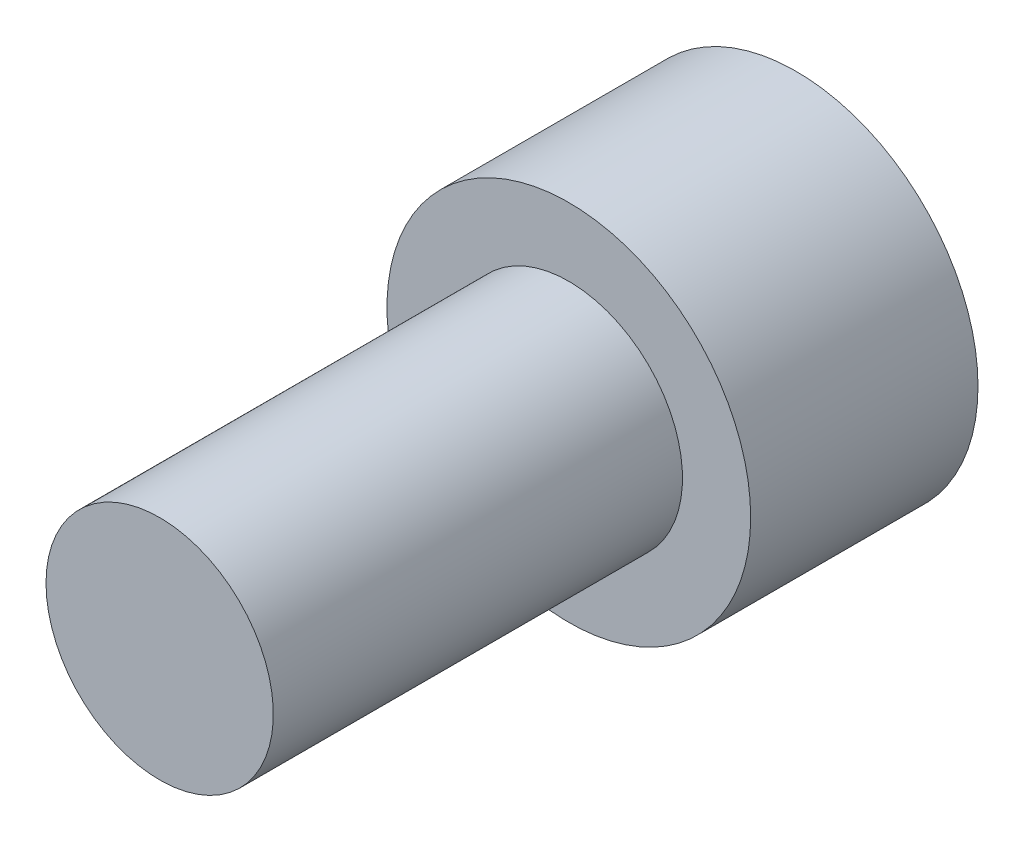
from build123d import *

# Parameters (mm, degrees)
SKETCH_1_R      = 20
EXTRUDE_1_DEPTH = 25
SKETCH_2_R      = 12.5
EXTRUDE_2_DEPTH = 45


with BuildPart() as part:
    # 草图1 → 凸台-拉伸1 (new body)
    with BuildSketch(Plane.XY):
        Circle(SKETCH_1_R)
    extrude(amount=EXTRUDE_1_DEPTH)

    # 草图2 → 凸台-拉伸2 (add)
    with BuildSketch(Plane.XY.offset(25)):
        with Locations(Location((0, 0, 0), (0, 0, 180))):
            Circle(SKETCH_2_R)
    extrude(amount=EXTRUDE_2_DEPTH)


solid = part.part
